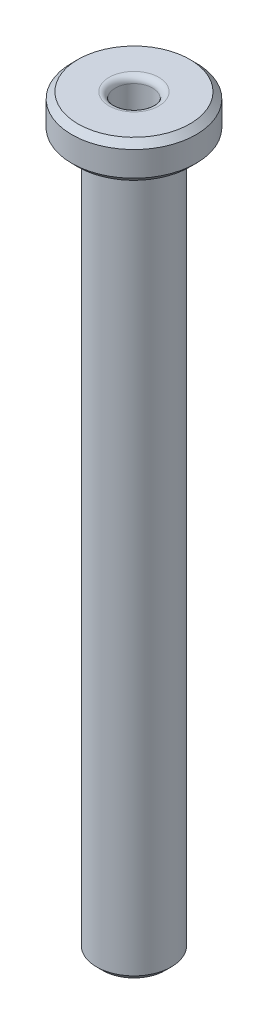
SolidWorks part; units mm, degrees
material "SKD11"
ref_plane "前视基准面" through (0, 0, 0) normal (0, 0, 1) x (1, 0, 0)
ref_plane "上视基准面" through (0, 0, 0) normal (0, 1, 0) x (1, 0, 0)
ref_plane "右视基准面" through (0, 0, 0) normal (1, 0, 0) x (0, 0, -1)
sketch "草图1" plane through (0, 0, 0) normal (0, 1, 0) x (1, 0, 0)
  circle A0 centre (0, 0) radius 3
  circle A1 centre (0, 0) radius 1.5
  dimension "D1" = 3
  dimension "D2" = 6
extrude "凸台-拉伸1" add sketch "草图1" along normal blind 60
sketch "草图2" plane through (0, 60, 0) normal (0, 1, 0) x (1, 0, 0)
  circle A0 centre (0, 0) radius 5
  circle A1 centre (0, 0) radius 1.5
  dimension "D1" = 10
  dimension "D2" = 3
extrude "凸台-拉伸2" add sketch "草图2" against normal blind 3
fillet "圆角1" radius 0.5 2 edges at (0, 60, 1.5) (0, 0, 1.5)
chamfer "倒角1" distance 0.5 angle 45 3 edges at (0, 57, 5) (0, 60, 5) (0, 0, 3)
